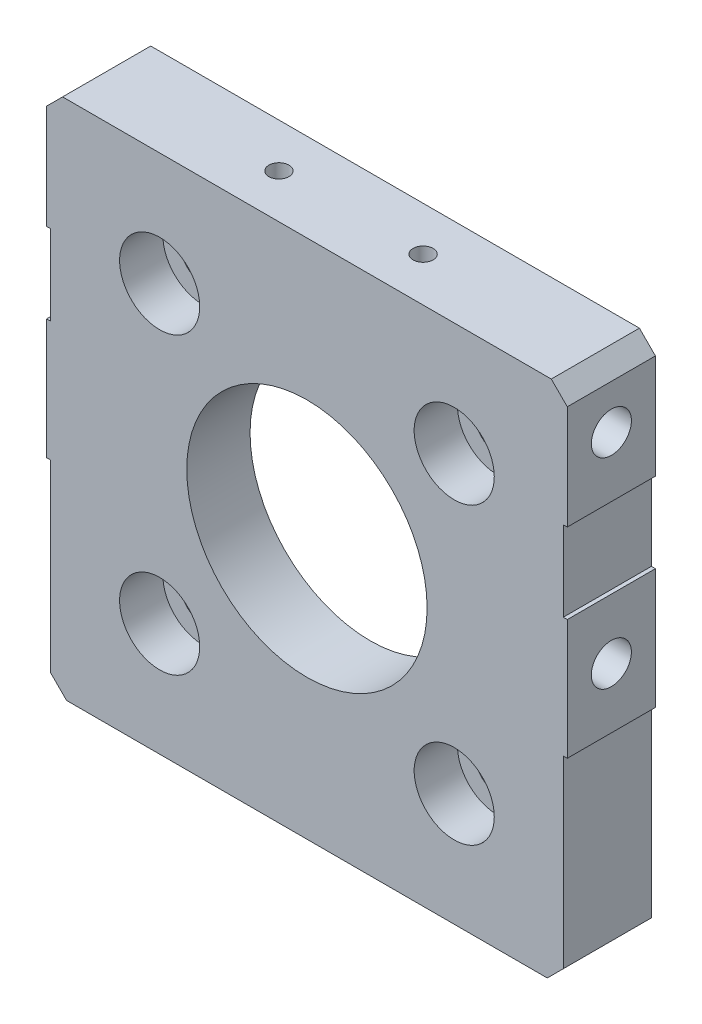
from build123d import *

# Parameters (mm, degrees)
SKETCH_1_W                   = 65
SKETCH_1_H                   = 65
EXTRUDE_1_DEPTH              = 5.5
SKETCH_3_R                   = 20.05
CUT_EXTRUDE_1_DEPTH          = 3.1
SKETCH_4_R                   = 15
CUT_EXTRUDE_2_DEPTH          = 47.635930354
HOLE_WIZARD_M5_1_D           = 5.5
HOLE_WIZARD_M5_1_CBORE_D     = 10
HOLE_WIZARD_M5_1_CBORE_DEPTH = 5.4
HOLE_WIZARD_M6_1_AT_2_COUNT  = 2
HOLE_WIZARD_M6_1_AT_2_PITCH  = 25
SKETCH_12_W                  = 11
SKETCH_12_H                  = 10
SKETCH_12_H_2                = 25
CUT_EXTRUDE_3_DEPTH          = 0.5
CHAMFER_1_SIZE               = 2
HOLE_WIZARD_M3_2_D           = 2.5
HOLE_WIZARD_M3_2_DEPTH       = 8.5
HOLE_WIZARD_M3_2_TIP         = 0.751075774
HOLE_WIZARD_M3_3_D           = 2.5
HOLE_WIZARD_M3_3_DEPTH       = 8.5
HOLE_WIZARD_M3_3_TIP         = 0.751075774


with BuildPart() as part:
    # 草图1 → 凸台-拉伸1 (new, symmetric)
    with BuildSketch(Plane.XY):
        Rectangle(SKETCH_1_W, SKETCH_1_H)
    extrude(amount=EXTRUDE_1_DEPTH, both=True)

    # 草图3 → 切除-拉伸1 (cut)
    with BuildSketch(Plane(origin=(0, 0, -5.5), x_dir=(-1, 0, 0), z_dir=(0, 0, -1))):
        Circle(SKETCH_3_R)
    extrude(amount=-CUT_EXTRUDE_1_DEPTH, mode=Mode.SUBTRACT)

    # 草图4 → 切除-拉伸2 (cut, through all)
    with BuildSketch(Plane(origin=(0, 0, -2.4), x_dir=(-1, 0, 0), z_dir=(0, 0, -1))):
        Circle(SKETCH_4_R)
    extrude(amount=-CUT_EXTRUDE_2_DEPTH, mode=Mode.SUBTRACT)

    # M5 六角凹头螺钉的柱形沉头孔1 (through all)
    with Locations(Plane.XY.offset(5.5)):
        with Locations((-18.384776311, 18.384776311), (18.384776311, 18.384776311), (18.384776311, -18.384776311), (-18.384776311, -18.384776311)):
            CounterBoreHole(HOLE_WIZARD_M5_1_D / 2, HOLE_WIZARD_M5_1_CBORE_D / 2, HOLE_WIZARD_M5_1_CBORE_DEPTH)

    # 草图8 → M6 螺纹孔1 (revolve, cut)
    with BuildSketch(Plane(origin=(-32.5, 0, 0), x_dir=(0, 0, 1), z_dir=(0, 1, 0))):
        Polygon((0, 0), (0, 11.502151548), (2.5, 10), (2.5, 0), align=None)
    hole_wizard_m6_1 = revolve(axis=Axis((-38.85, 0, 0), (1, 0, 0)), mode=Mode.SUBTRACT)

    # M6 螺纹孔1 at 2: M6 螺纹孔1 ×2
    with Locations(*[(0, i * HOLE_WIZARD_M6_1_AT_2_PITCH, 0) for i in range(1, HOLE_WIZARD_M6_1_AT_2_COUNT)]):
        add(hole_wizard_m6_1, mode=Mode.SUBTRACT)

    # 草图12 → 切除-拉伸3 (cut)
    with BuildSketch(Plane.ZY.offset(32.5)):
        with Locations((0, 12.5)):
            Rectangle(SKETCH_12_W, SKETCH_12_H)
        with Locations((0, -20)):
            Rectangle(SKETCH_12_W, SKETCH_12_H_2)
    cut_extrude_3 = extrude(amount=-CUT_EXTRUDE_3_DEPTH, mode=Mode.SUBTRACT)

    # 镜向1: M6 螺纹孔1, 切除-拉伸3 across plane
    add(hole_wizard_m6_1.mirror(Plane(origin=(0, 0, 0), x_dir=(0, 0, 1), z_dir=(1, 0, 0))), mode=Mode.SUBTRACT)
    add(cut_extrude_3.mirror(Plane(origin=(0, 0, 0), x_dir=(0, 0, 1), z_dir=(1, 0, 0))), mode=Mode.SUBTRACT)

    # 镜向1 copy 1 sketch → 镜向1 copy 1 (revolve, cut)
    with BuildSketch(Plane(origin=(32.5, 25, 0), x_dir=(0, 0, 1), z_dir=(0, 1, 0))):
        Polygon((0, 0), (0, -11.502151548), (2.5, -10), (2.5, 0), align=None)
    revolve(axis=Axis((38.85, 25, 0), (1, 0, 0)), mode=Mode.SUBTRACT)

    # 倒角1
    chamfer_1_edges = [part.edges().sort_by_distance(p)[0] for p in [
        (32, -32.5, 0),
        (-32.5, 32.5, 0),
        (32.5, 32.5, 0),
        (-32, -32.5, 0),
    ]]
    chamfer(chamfer_1_edges, length=CHAMFER_1_SIZE)

    # M3 螺纹孔2
    with Locations(Plane(origin=(0, 32.5, 0), x_dir=(1, 0, 0), z_dir=(0, 1, 0))):
        with Locations((-9, 0), (9, 0)):
            Hole(HOLE_WIZARD_M3_2_D / 2, depth=HOLE_WIZARD_M3_2_DEPTH)
            with Locations((0, 0, -(HOLE_WIZARD_M3_2_DEPTH + HOLE_WIZARD_M3_2_TIP / 2))):  # 118° drill point
                Cone(0, HOLE_WIZARD_M3_2_D / 2, HOLE_WIZARD_M3_2_TIP, mode=Mode.SUBTRACT)

    # M3 螺纹孔3
    with Locations(Plane(origin=(0, -32.5, 0), x_dir=(-1, 0, 0), z_dir=(0, -1, 0))):
        with Locations((-9, 1.25), (9, 1.25)):
            Hole(HOLE_WIZARD_M3_3_D / 2, depth=HOLE_WIZARD_M3_3_DEPTH)
            with Locations((0, 0, -(HOLE_WIZARD_M3_3_DEPTH + HOLE_WIZARD_M3_3_TIP / 2))):  # 118° drill point
                Cone(0, HOLE_WIZARD_M3_3_D / 2, HOLE_WIZARD_M3_3_TIP, mode=Mode.SUBTRACT)


solid = part.part
